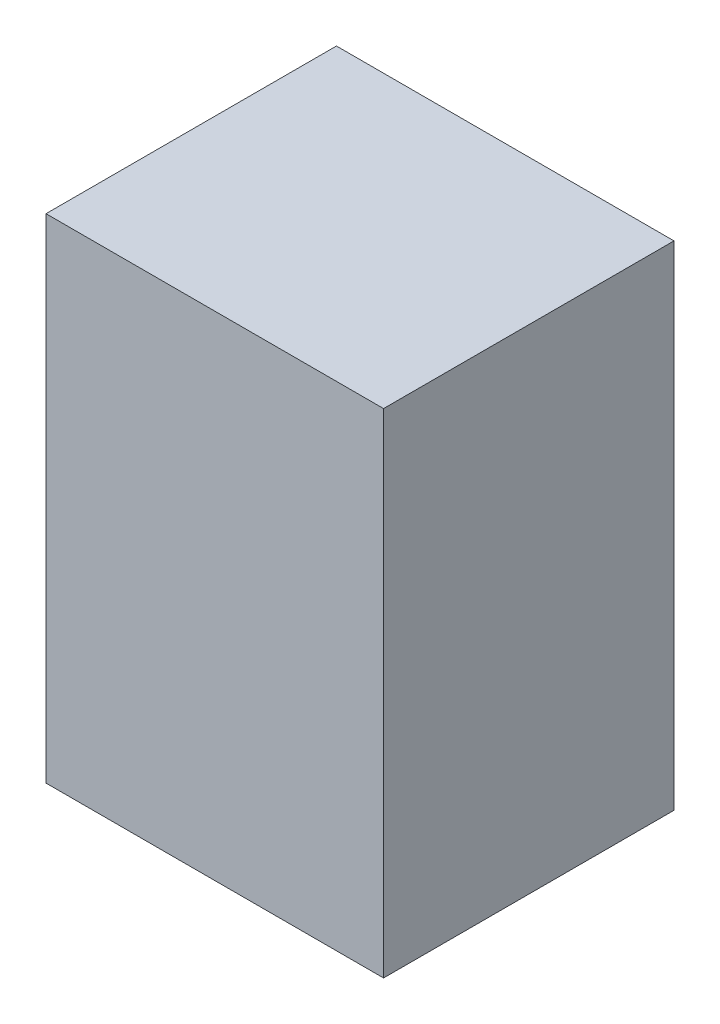
SolidWorks part; units mm, degrees
ref_plane "Front Plane" through (0, 0, 0) normal (0, 0, 1) x (1, 0, 0)
ref_plane "Top Plane" through (0, 0, 0) normal (0, 1, 0) x (1, 0, 0)
ref_plane "Right Plane" through (0, 0, 0) normal (1, 0, 0) x (0, 0, -1)
sketch "Sketch1" plane through (0, 0, 0) normal (0, 0, 1) x (1, 0, 0)
  line L1 (-17.4331, 25.4698) -> (17.4331, 25.4698)
  line L2 (-17.4331, 25.4698) -> (-17.4331, -25.4698)
  line L3 (-17.4331, -25.4698) -> (17.4331, -25.4698)
  line L4 (17.4331, 25.4698) -> (17.4331, -25.4698)
  line L5 (-17.4331, 25.4698) -> (17.4331, -25.4698) construction
  line L6 (-17.4331, -25.4698) -> (17.4331, 25.4698) construction
  point P0 (0, 0)
extrude "Boss-Extrude1" add sketch "Sketch1" against normal blind 30
